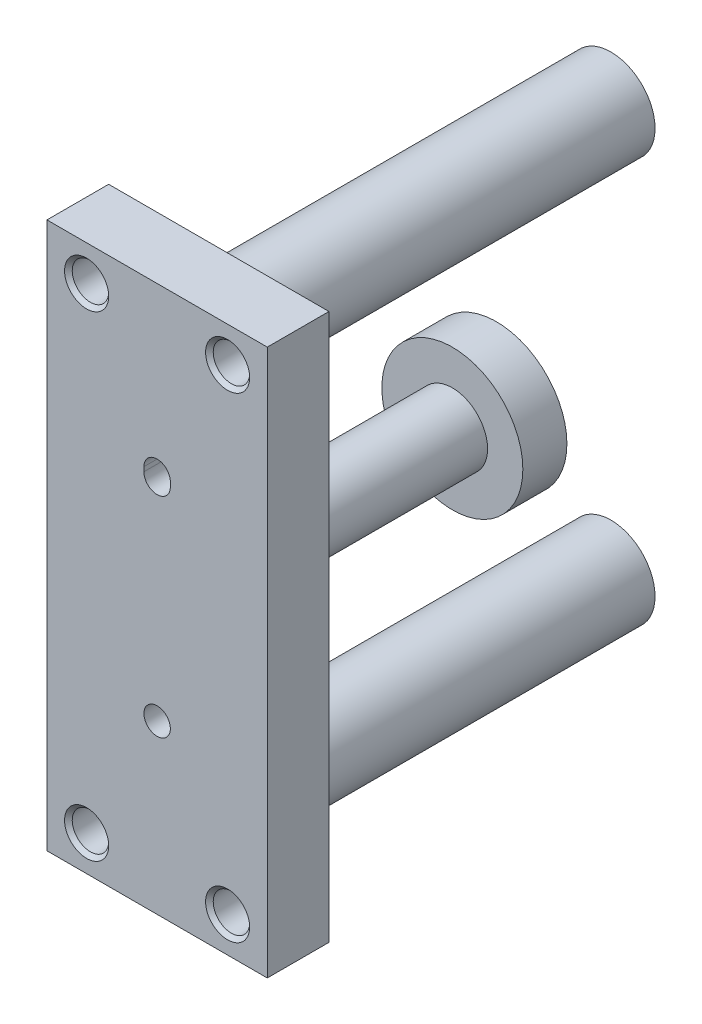
from build123d import *

# Parameters (mm, degrees)
SKETCH1_W           = 25
SKETCH1_H           = 62
BOSS_EXTRUDE1_DEPTH = 7
SKETCH2_R           = 5
BOSS_EXTRUDE2_DEPTH = 56
SKETCH3_R           = 5
BOSS_EXTRUDE3_DEPTH = 56
HOLE1_D             = 3
HOLE1_DEPTH         = 6
HOLE1_TIP           = 0.866025404
CUT_EXTRUDE1_DEPTH  = 3
HOLE2_D             = 3
HOLE2_DEPTH         = 6
HOLE2_TIP           = 0.866025404
SKETCH14_W          = 10
SKETCH14_H          = 56
CUT_EXTRUDE2_DEPTH  = 4.5


with BuildPart() as part:
    # Sketch1 → Boss-Extrude1 (new body)
    with BuildSketch(Plane.XY.offset(13)):
        Rectangle(SKETCH1_W, SKETCH1_H)
    extrude(amount=-BOSS_EXTRUDE1_DEPTH)

    # Sketch2 → Boss-Extrude2 (add)
    with BuildSketch(Plane.XY.offset(13)):
        with Locations((0, 23)):
            Circle(SKETCH2_R)
    extrude(amount=-BOSS_EXTRUDE2_DEPTH)

    # Sketch3 → Boss-Extrude3 (add)
    with BuildSketch(Plane.XY.offset(13)):
        with Locations((0, -23)):
            Circle(SKETCH3_R)
    extrude(amount=-BOSS_EXTRUDE3_DEPTH)

    # Sketch4 → Revolve1 (revolve)
    with BuildSketch(Plane(origin=(0, 0, 0), x_dir=(0, 0, -1), z_dir=(1, 0, 0)), mode=Mode.PRIVATE) as revolve1_sk:
        Polygon((-6, 0), (-6, 4), (20.5, 4), (20.5, 8), (25.5, 8), (25.5, 0), align=None)
    revolve(revolve1_sk.sketch.rotate(Axis((0, 0, -25.5), (0, 0, 1)), 270), axis=Axis((0, 0, -25.5), (0, 0, 1)))

    # Hole1
    with Locations(Plane.XY.offset(13)):
        with Locations((0, 12)):
            Hole(HOLE1_D / 2, depth=HOLE1_DEPTH)
            with Locations((0, 0, -(HOLE1_DEPTH + HOLE1_TIP / 2))):  # 120° drill point
                Cone(0, HOLE1_D / 2, HOLE1_TIP, mode=Mode.SUBTRACT)

    # Sketch7 → Cut-Extrude1 (cut)
    with BuildSketch(Plane.XY.offset(13)):
        with BuildLine():
            Line((1.5, 11.75), (1.5, 12.25))
            ThreePointArc((1.5, 12.25), (0, 13.75), (-1.5, 12.25))
            Line((-1.5, 12.25), (-1.5, 11.75))
            ThreePointArc((-1.5, 11.75), (0, 10.25), (1.5, 11.75))
        make_face()
    extrude(amount=-CUT_EXTRUDE1_DEPTH, mode=Mode.SUBTRACT)

    # Hole2
    with Locations(Plane.XY.offset(13)):
        with Locations((0, -12)):
            Hole(HOLE2_D / 2, depth=HOLE2_DEPTH)
            with Locations((0, 0, -(HOLE2_DEPTH + HOLE2_TIP / 2))):  # 120° drill point
                Cone(0, HOLE2_D / 2, HOLE2_TIP, mode=Mode.SUBTRACT)

    # Sketch10 → Cut-Revolve1 (revolve, cut)
    with BuildSketch(Plane(origin=(0, -27, 0), x_dir=(1, 0, 0), z_dir=(0, 1, 0)), mode=Mode.PRIVATE) as cut_revolve1_sk:
        Polygon((8, -6), (10.5, -6), (10.067, -6.433), (10.067, -12.567), (10.5, -13), (8, -13), align=None)
    revolve(cut_revolve1_sk.sketch.rotate(Axis((8, -27, 13), (0, 0, -1)), 180), axis=Axis((8, -27, 13), (0, 0, -1)), mode=Mode.SUBTRACT)

    # Sketch11 → Cut-Revolve2 (revolve, cut)
    with BuildSketch(Plane(origin=(0, -27, 0), x_dir=(1, 0, 0), z_dir=(0, 1, 0)), mode=Mode.PRIVATE) as cut_revolve2_sk:
        Polygon((-8, -6), (-5.5, -6), (-5.933, -6.433), (-5.933, -12.567), (-5.5, -13), (-8, -13), align=None)
    revolve(cut_revolve2_sk.sketch.rotate(Axis((-8, -27, 13), (0, 0, -1)), 180), axis=Axis((-8, -27, 13), (0, 0, -1)), mode=Mode.SUBTRACT)

    # Sketch12 → Cut-Revolve3 (revolve, cut)
    with BuildSketch(Plane(origin=(0, 27, 0), x_dir=(1, 0, 0), z_dir=(0, 1, 0)), mode=Mode.PRIVATE) as cut_revolve3_sk:
        Polygon((8, -6), (10.5, -6), (10.067, -6.433), (10.067, -12.567), (10.5, -13), (8, -13), align=None)
    revolve(cut_revolve3_sk.sketch.rotate(Axis((8, 27, 13), (0, 0, -1)), 180), axis=Axis((8, 27, 13), (0, 0, -1)), mode=Mode.SUBTRACT)

    # Sketch13 → Cut-Revolve4 (revolve, cut)
    with BuildSketch(Plane(origin=(0, 27, 0), x_dir=(1, 0, 0), z_dir=(0, 1, 0)), mode=Mode.PRIVATE) as cut_revolve4_sk:
        Polygon((-8, -6), (-5.5, -6), (-5.933, -6.433), (-5.933, -12.567), (-5.5, -13), (-8, -13), align=None)
    revolve(cut_revolve4_sk.sketch.rotate(Axis((-8, 27, 13), (0, 0, -1)), 180), axis=Axis((-8, 27, 13), (0, 0, -1)), mode=Mode.SUBTRACT)

    # Sketch14 → Cut-Extrude2 (cut)
    with BuildSketch(Plane(origin=(0, 0, -43), x_dir=(-1, 0, 0), z_dir=(0, 0, -1))):
        Rectangle(SKETCH14_W, SKETCH14_H)
    extrude(amount=-CUT_EXTRUDE2_DEPTH, mode=Mode.SUBTRACT)


solid = part.part
